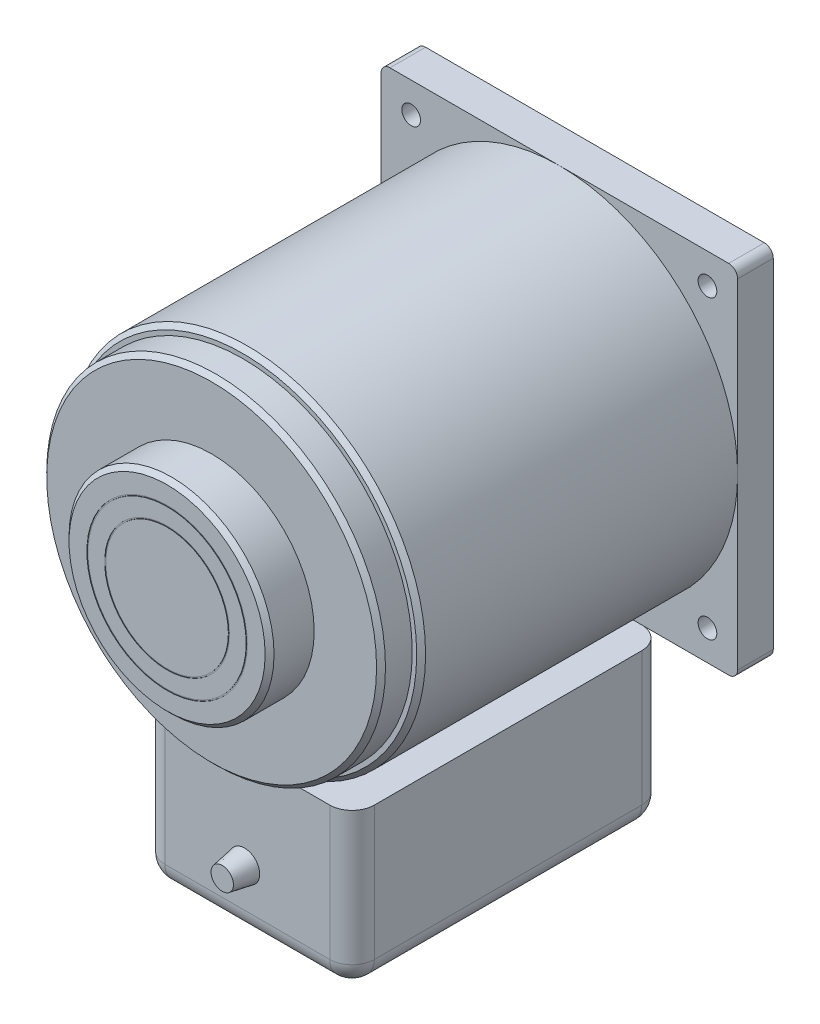
SolidWorks part; units mm, degrees
ref_plane "前视基准面" through (0, 0, 0) normal (0, 0, 1) x (1, 0, 0)
ref_plane "上视基准面" through (0, 0, 0) normal (0, 1, 0) x (1, 0, 0)
ref_plane "右视基准面" through (0, 0, 0) normal (1, 0, 0) x (0, 0, -1)
sketch "草图1" plane through (0, 0, 0) normal (0, 0, 1) x (1, 0, 0)
  line L1 (0, 0) -> (80, 0)
  line L2 (0, 0) -> (0, 80)
  line L3 (0, 80) -> (80, 80)
  line L4 (80, 0) -> (80, 80)
  dimension "D1" = 80
  dimension "D2" = 80
extrude "凸台-拉伸1" add sketch "草图1" along normal blind 8
sketch "草图2" plane through (0, 0, 8) normal (0, 0, 1) x (1, 0, 0)
  line L0 (80, 80) -> (0, 80) construction
  line L1 (80, 0) -> (80, 80) construction
  circle A0 centre (40, 40) radius 40
  dimension "D1" = 80
  dimension "D2" = 40
  dimension "D3" = 40
extrude "凸台-拉伸2" add sketch "草图2" along normal blind 71
sketch "草图3" plane through (0, 0, 79) normal (0, 0, 1) x (1, 0, 0)
  circle A0 centre (40, 40) radius 38
  dimension "D1" = 76
extrude "凸台-拉伸3" add sketch "草图3" along normal blind 7
sketch "草图4" plane through (0, 0, 86) normal (0, 0, 1) x (1, 0, 0)
  circle A0 centre (40, 40) radius 23
  dimension "D1" = 46
extrude "凸台-拉伸4" add sketch "草图4" along normal blind 10
sketch "草图5" plane through (0, 0, 0) normal (0, 0, -1) x (-1, 0, 0)
  line L0 (-80, 0) -> (-80, 80) construction
  line L1 (0, 0) -> (-80, 0) construction
  circle A0 centre (-40, 40) radius 4
  dimension "D1" = 8
  dimension "D2" = 40
  dimension "D3" = 40
extrude "凸台-拉伸5" add sketch "草图5" along normal blind 20
fillet "圆角1" radius 2 4 edges at (80, 0, 4) (0, 0, 4) (0, 80, 4) (80, 80, 4)
chamfer "倒角1" distance 1 angle 45 3 edges at (63, 40, 96) (78, 40, 86) (80, 40, 79)
sketch "草图6" plane through (0, 0, 96) normal (0, 0, 1) x (1, 0, 0)
  circle A0 centre (40, 40) radius 18
  circle A1 centre (40, 40) radius 14
  circle A2 centre (40, 40) radius 17.75
  circle A3 centre (40, 40) radius 13.75
  dimension "D1" = 36
  dimension "D2" = 28
  dimension "D3" = 35.5
  dimension "D4" = 27.5
extrude "切除-拉伸2" cut sketch "草图6" against normal blind 0.1 contours A0 | A2 | A3 | A1
sketch "草图8" plane through (0, 0, 8) normal (0, 0, 1) x (1, 0, 0)
  line L0 (40, 0) -> (78, 0) construction
  line L1 (63.5, 0) -> (16.5, 0)
  line L2 (16.5, 0) -> (16.5, -35)
  line L3 (16.5, -35) -> (63.5, -35)
  line L4 (63.5, -35) -> (63.5, 0)
  line L6 (0, 40) -> (0, 2) construction
  dimension "D1" = 16.5
  dimension "D2" = 47
  dimension "D3" = 35
extrude "凸台-拉伸6" add sketch "草图8" along normal blind 70
fillet "圆角2" radius 5 8 edges at (16.5, -17.5, 8) (16.5, -17.5, 78) (63.5, -17.5, 78) (63.5, -17.5, 8) (16.5, -35, 43) (40, -35, 78) (63.5, -35, 43) (40, -35, 8)
sketch "草图9" plane through (0, 0, 78) normal (0, 0, 1) x (1, 0, 0)
  circle A0 centre (39.3776, -21.3001) radius 3.3983
extrude "凸台-拉伸7" add sketch "草图9" along normal blind 5 draft 10
sketch "草图12" plane through (0, 0, 0) normal (0, 0, -1) x (-1, 0, 0)
  line L1 (-78, 2) -> (-73.234, 6.766) construction
  line L2 (-78, 78) -> (-73.234, 73.234) construction
  line L4 (-6.766, 6.766) -> (-2, 2) construction
  line L5 (-6.766, 73.234) -> (-2, 78) construction
hole_wizard "M5 螺纹孔1" positions "3D草图1" profile "草图13" tap size "M5" standard "Iso" end condition through all
sketch3d "3D草图1"
  point P0 (73.234, 73.234, 0)
  point P3 (6.766, 73.234, 0)
  point P6 (6.766, 6.766, 0)
  point P9 (73.234, 6.766, 0)
sketch "草图13" plane through (73.234, 73.234, 0) normal (1, 0, 0) x (0, 1, 0)
  line L0 (0, 0) -> (0, 96)
  line L1 (0, 96) -> (2.1, 96)
  line L2 (2.1, 96) -> (2.1, 0)
  line L5 (2.1, 0) -> (0, 0)
  line L11 (0, -6.35) -> (0, 107.95) construction
  dimension "通孔螺纹孔钻头直径" = 4.2
  dimension "通孔螺纹孔钻头深度" = 96
cosmetic thread "孔螺蚊线1" parameters "D2"=5
cosmetic thread "孔螺蚊线2" parameters "D2"=5
cosmetic thread "孔螺蚊线3" parameters "D2"=5
cosmetic thread "孔螺蚊线4" parameters "D2"=5
